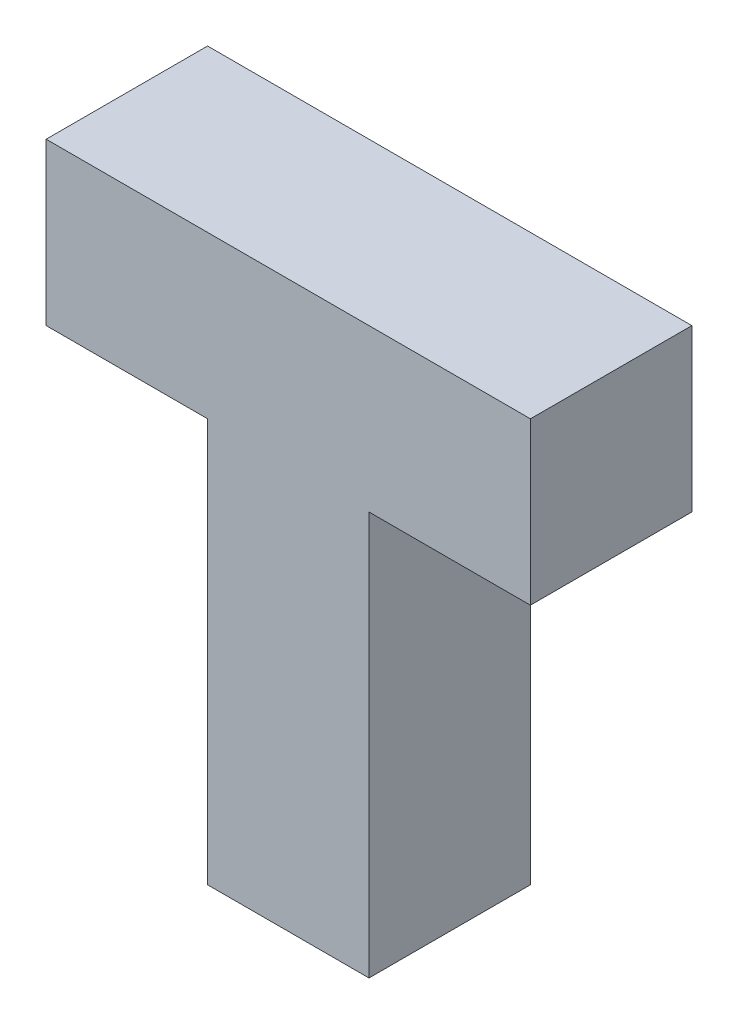
SolidWorks part; units mm, degrees
ref_plane "Front Plane" through (0, 0, 0) normal (0, 0, 1) x (1, 0, 0)
ref_plane "Top Plane" through (0, 0, 0) normal (0, 1, 0) x (1, 0, 0)
ref_plane "Right Plane" through (0, 0, 0) normal (1, 0, 0) x (0, 0, -1)
sketch "Sketch1" plane through (0, 0, 0) normal (0, 0, 1) x (1, 0, 0)
  line L0 (-15, 17.5) -> (15, -17.5) construction
  line L1 (-15, 17.5) -> (15, 17.5)
  line L2 (-15, 17.5) -> (-15, -17.5)
  line L3 (-15, -17.5) -> (15, -17.5)
  line L4 (15, 17.5) -> (15, -17.5)
  dimension "D1" = 30
  dimension "D2" = 35
extrude "Boss-Extrude1" add sketch "Sketch1" along normal blind 10
sketch "Sketch2" plane through (0, 0, 10) normal (0, 0, 1) x (1, 0, 0)
  line L0 (15, 17.5) -> (-15, 17.5) construction
  line L1 (-15, -17.5) -> (-5, -17.5)
  line L2 (-15, -17.5) -> (-15, 7.5)
  line L3 (-15, 7.5) -> (-5, 7.5)
  line L4 (-5, -17.5) -> (-5, 7.5)
  line L5 (15, -17.5) -> (5, -17.5)
  line L6 (15, -17.5) -> (15, 7.5)
  line L7 (15, 7.5) -> (5, 7.5)
  line L8 (5, -17.5) -> (5, 7.5)
  dimension "D1" = 10
  dimension "D2" = 10
extrude "Cut-Extrude1" cut sketch "Sketch2" against normal through all
